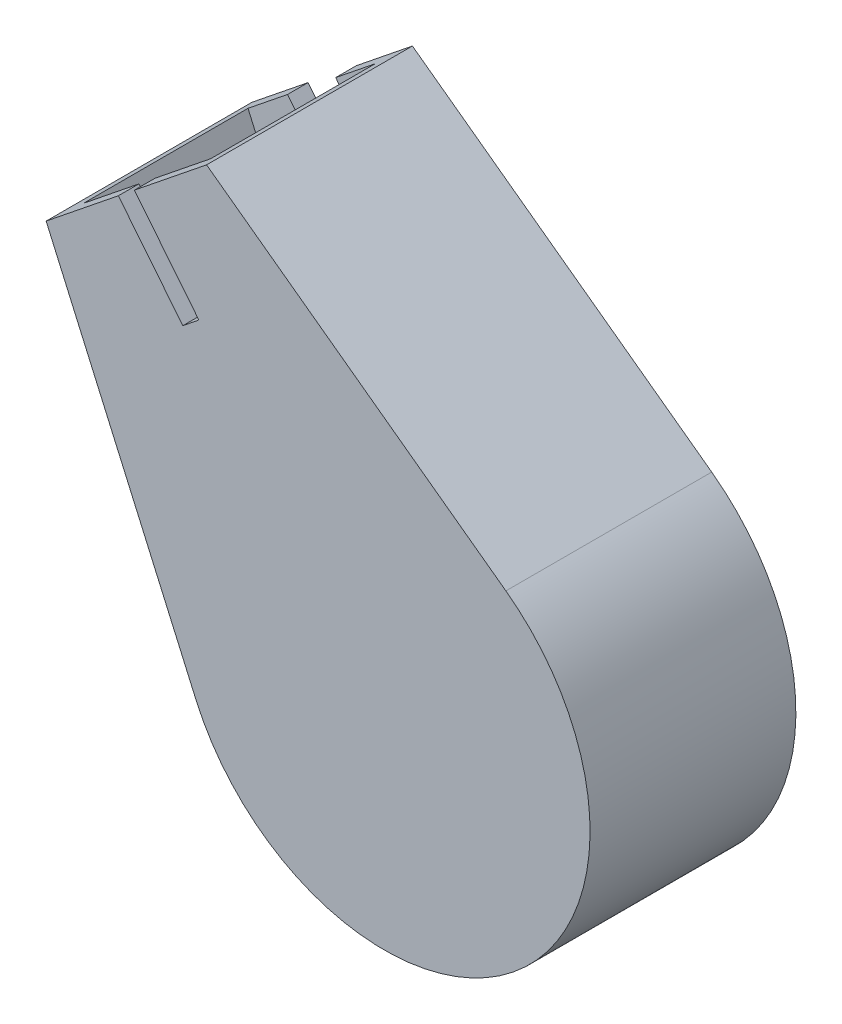
SolidWorks part; units mm, degrees
ref_plane "Front Plane" through (0, 0, 0) normal (0, 0, 1) x (1, 0, 0)
ref_plane "Top Plane" through (0, 0, 0) normal (0, 1, 0) x (1, 0, 0)
ref_plane "Right Plane" through (0, 0, 0) normal (1, 0, 0) x (0, 0, -1)
other "Configuration Table"
sketch "Sketch1" plane through (0, 0, 0) normal (0, 0, 1) x (1, 0, 0)
  line L0 (-18.2983, -8.0729) -> (-32.852, 24.9148)
  line L1 (-17.2624, 37.4434) -> (11.8211, 16.1326)
  line L2 (0, 0) -> (-25.0572, 31.1791) construction
  line L5 (-32.852, 24.9148) -> (-17.2624, 37.4434)
  circle A0 centre (0, 0) radius 20
  circle A1 centre (0, 0) radius 20 construction
  dimension "D2" = 40
  dimension "D1" = 40
  dimension "D3" = 20
extrude "Boss-Extrude1" add sketch "Sketch1" along normal blind 20
shell "Shell1" thickness 2
sketch "Sketch2" plane through (0, 0, 0) normal (0, 0, -1) x (-1, 0, 0)
  line L0 (21.1313, 21.505) -> (16.4545, 25.2636)
  line L1 (21.1313, 21.505) -> (33.6599, 37.0946)
  line L2 (16.4545, 25.2636) -> (28.9831, 40.8532)
  line L3 (33.6599, 37.0946) -> (28.9831, 40.8532)
  line L4 (21.1313, 21.505) -> (28.9831, 40.8532) construction
  line L5 (16.4545, 25.2636) -> (33.6599, 37.0946) construction
  line L6 (32.852, 24.9148) -> (17.2624, 37.4434) construction
  point P1 (25.0572, 31.1791)
  point P3 (25.0572, 31.1791)
  dimension "D1" = 6
  dimension "D2" = 10
extrude "Cut-Extrude1" cut sketch "Sketch2" against normal up to next
sketch "Sketch3" plane through (0, 0, 20) normal (0, 0, 1) x (1, 0, 0)
  line L4 (-18.0119, 24.0088) -> (-512.5668, 639.3918)
  line L5 (-512.5668, 639.3918) -> (-514.1257, 638.139)
  line L6 (-514.1257, 638.139) -> (-19.5708, 22.756)
  line L7 (-19.5708, 22.756) -> (-18.0119, 24.0088)
  line L8 (-18.0119, 24.0088) -> (-512.5668, 639.3918)
  line L9 (-512.5668, 639.3918) -> (-514.1257, 638.139)
  line L10 (-514.1257, 638.139) -> (-19.5708, 22.756)
  line L11 (-19.5708, 22.756) -> (-18.0119, 24.0088)
  dimension "D1" = 0
extrude "Cut-Extrude2" cut sketch "Sketch3" against normal up to surface (18 mm away)
